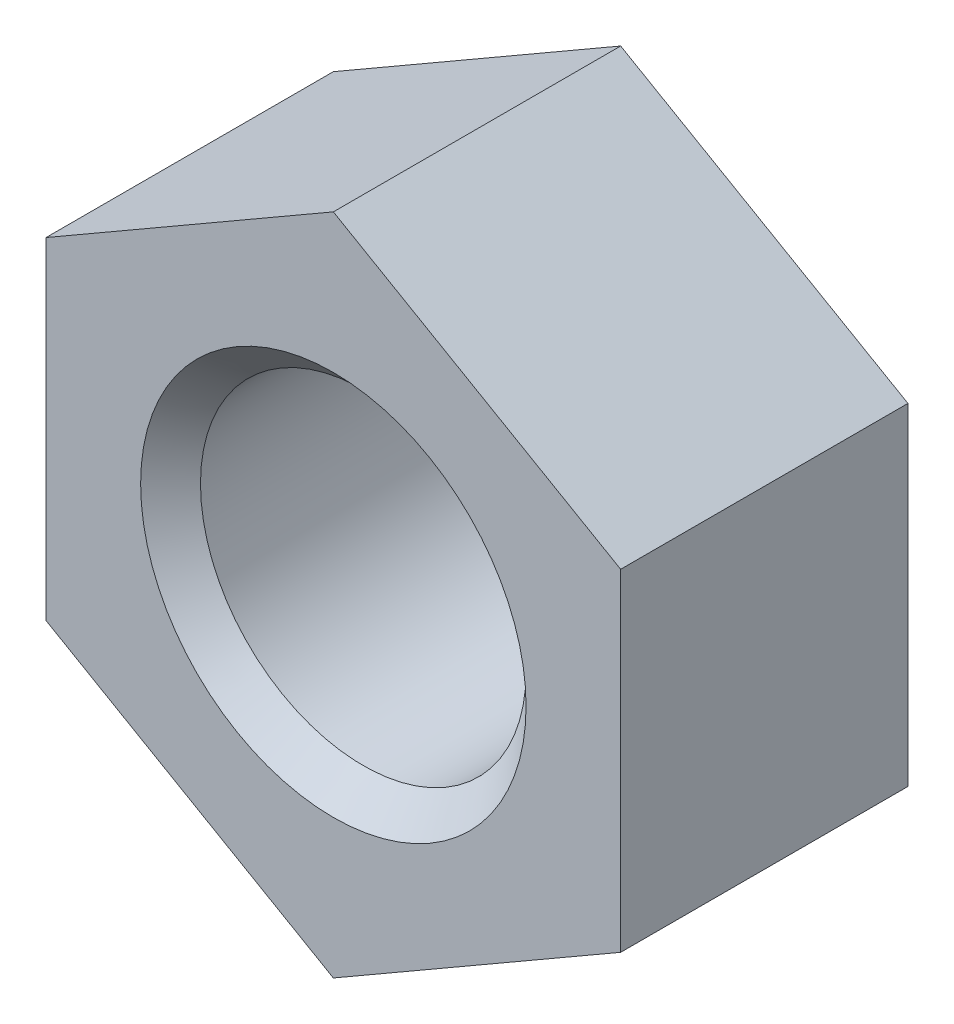
from build123d import *

# Parameters (mm, degrees)
BOSS_EXTRUDE1_DEPTH         = 6
M8_TAPPED_HOLE1_D           = 6.8
M8_TAPPED_HOLE1_CSINK_D     = 8.05
M8_TAPPED_HOLE1_CSINK_ANGLE = 90


with BuildPart() as part:
    # Sketch1 → Boss-Extrude1 (new body)
    with BuildSketch(Plane.XY):
        Polygon((-5.093902669, -2.715310597), (-5.093902669, 4.212892633), (0.906097331, 7.676994248), (6.906097331, 4.212892633), (6.906097331, -2.715310597), (0.906097331, -6.179412212), align=None)
    extrude(amount=BOSS_EXTRUDE1_DEPTH)

    # M8 Tapped Hole1 (through all)
    with Locations(Plane.XY.offset(6)):
        with Locations((0.906097331, 0.748791018)):
            CounterSinkHole(M8_TAPPED_HOLE1_D / 2, M8_TAPPED_HOLE1_CSINK_D / 2, counter_sink_angle=M8_TAPPED_HOLE1_CSINK_ANGLE)


solid = part.part
